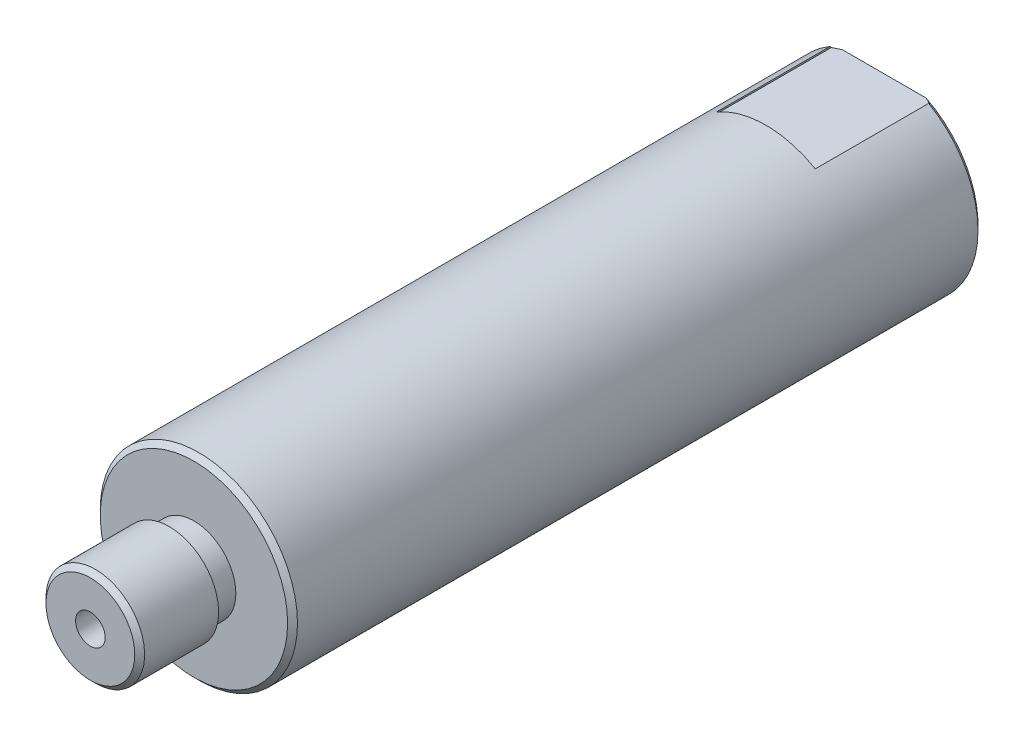
from build123d import *

# Parameters (mm, degrees)
SKETCH_1_R                 = 10
EXTRUDE_1_DEPTH            = 70
SKETCH_2_R                 = 5
EXTRUDE_2_DEPTH            = 10.5
SKETCH_3_W                 = 0.75
SKETCH_3_H                 = 2.5
SKETCH_4_R                 = 1.5
CUT_EXTRUDE_1_DEPTH        = 15.5
HOLE_WIZARD_6_0_6_1_REACH  = 68.521
HOLE_WIZARD_6_0_6_1_BORE_R = 3
CHAMFER_1_SIZE             = 0.5
SKETCH_9_W                 = 10
SKETCH_9_H                 = 12
CUT_EXTRUDE_2_DEPTH        = 1.5


with BuildPart() as part:
    # 草图1 → 凸台-拉伸1 (new body)
    with BuildSketch(Plane.XY):
        Circle(SKETCH_1_R)
    extrude(amount=EXTRUDE_1_DEPTH)

    # 草图2 → 凸台-拉伸2 (add)
    with BuildSketch(Plane.XY.offset(70)):
        with Locations(Location((0, 0, 0), (0, 0, 180))):
            Circle(SKETCH_2_R)
    extrude(amount=EXTRUDE_2_DEPTH)

    # 草图3 → 切除-旋转1 (revolve, cut)
    with BuildSketch(Plane(origin=(0, 0, 0), x_dir=(1, 0, 0), z_dir=(0, 1, 0)), mode=Mode.PRIVATE) as cut_revolve_1_sk:
        with Locations((-4.625, -71.25)):
            Rectangle(SKETCH_3_W, SKETCH_3_H)
    revolve(cut_revolve_1_sk.sketch.rotate(Axis((0, 0, 80.5), (0, 0, -1)), 180), axis=Axis((0, 0, 80.5), (0, 0, -1)), mode=Mode.SUBTRACT)

    # 草图4 → 切除-拉伸1 (cut)
    with BuildSketch(Plane.XY.offset(80.5)):
        Circle(SKETCH_4_R)
    extrude(amount=-CUT_EXTRUDE_1_DEPTH, mode=Mode.SUBTRACT)

    # 草图5 → 1/4 NPT 螺纹孔1 (revolve, cut)
    with BuildSketch(Plane.YZ):
        Polygon((0, 0), (0, 20.412347279), (5.5626, 17.07), (5.5626, 10.02), (5.943676082, 10.02), (6.2436883, 0), align=None)
    revolve(axis=Axis((0, 0, -6.35), (0, 0, 1)), mode=Mode.SUBTRACT)

    # Ø6.0 (6) 直径孔1 bore → Ø6.0 (6) 直径孔1 (cut, up to next)
    with BuildSketch(Plane.XY.offset(65), mode=Mode.PRIVATE) as hole_wizard_6_0_6_1_sk1:
        Circle(HOLE_WIZARD_6_0_6_1_BORE_R)
    hole_wizard_6_0_6_1_tool1 = extrude(hole_wizard_6_0_6_1_sk1.sketch, amount=-HOLE_WIZARD_6_0_6_1_REACH, mode=Mode.PRIVATE) & part.part
    add(hole_wizard_6_0_6_1_tool1.solids().sort_by_distance((0, 0, 65))[0], mode=Mode.SUBTRACT)

    # 倒角1
    chamfer_1_edges = [part.edges().sort_by_distance(p)[0] for p in [
        (-10, 0, 0),
        (-10, 0, 70),
        (5, 0, 80.5),
    ]]
    chamfer(chamfer_1_edges, length=CHAMFER_1_SIZE)

    # 草图9 → 切除-拉伸2 (cut)
    with BuildSketch(Plane(origin=(0, 10, 0), x_dir=(1, 0, 0), z_dir=(0, 1, 0))):
        with Locations((0, -6)):
            Rectangle(SKETCH_9_W, SKETCH_9_H)
    cut_extrude_2 = extrude(amount=-CUT_EXTRUDE_2_DEPTH, mode=Mode.SUBTRACT)

    # 镜向1: 切除-拉伸2 across plane
    add(cut_extrude_2.mirror(Plane.ZX), mode=Mode.SUBTRACT)


solid = part.part
